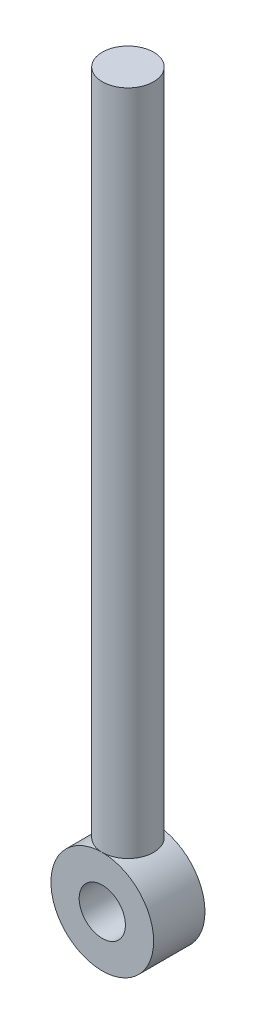
SolidWorks part; units mm, degrees
material "K"
ref_plane "Front" through (0, 0, 0) normal (0, 0, 1) x (1, 0, 0)
ref_plane "Top" through (0, 0, 0) normal (0, 1, 0) x (1, 0, 0)
ref_plane "Right" through (0, 0, 0) normal (1, 0, 0) x (0, 0, -1)
sketch "Sketch1" plane through (0, 0, 0) normal (0, 0, 1) x (1, 0, 0)
  circle A0 centre (0, 0) radius 10
  dimension "D1" = 20
extrude "Boss-Extrude1" add sketch "Sketch1" along normal mid plane 10
sketch "Sketch2" plane through (0, 0, 5) normal (0, 0, 1) x (1, 0, 0)
  circle A0 centre (0, 0) radius 4.5
  dimension "D1" = 9
extrude "Cut-Extrude1" cut sketch "Sketch2" against normal blind 10 contours A0
sketch "Sketch4" plane through (0, 0, 0) normal (0, 0, 1) x (1, 0, 0)
  line L0 (0, 10) -> (0, 140)
  line L1 (0, 140) -> (5, 140)
  line L2 (5, 140) -> (5, 10)
  line L3 (5, 10) -> (0, 10)
  circle A0 centre (0, 0) radius 10 construction
  dimension "D1" = 5
  dimension "D2" = 130
revolve "Revolve1" add sketch "Sketch4" angle 360 about L0
cosmetic thread "Cosmetic Thread1" parameters "D1"=110, "D2"=9
equation "\"零件重量\"= IIF ( \"SW-质量\" > 100 , int ( \"SW-质量\" ) , \"SW-质量\" )"
